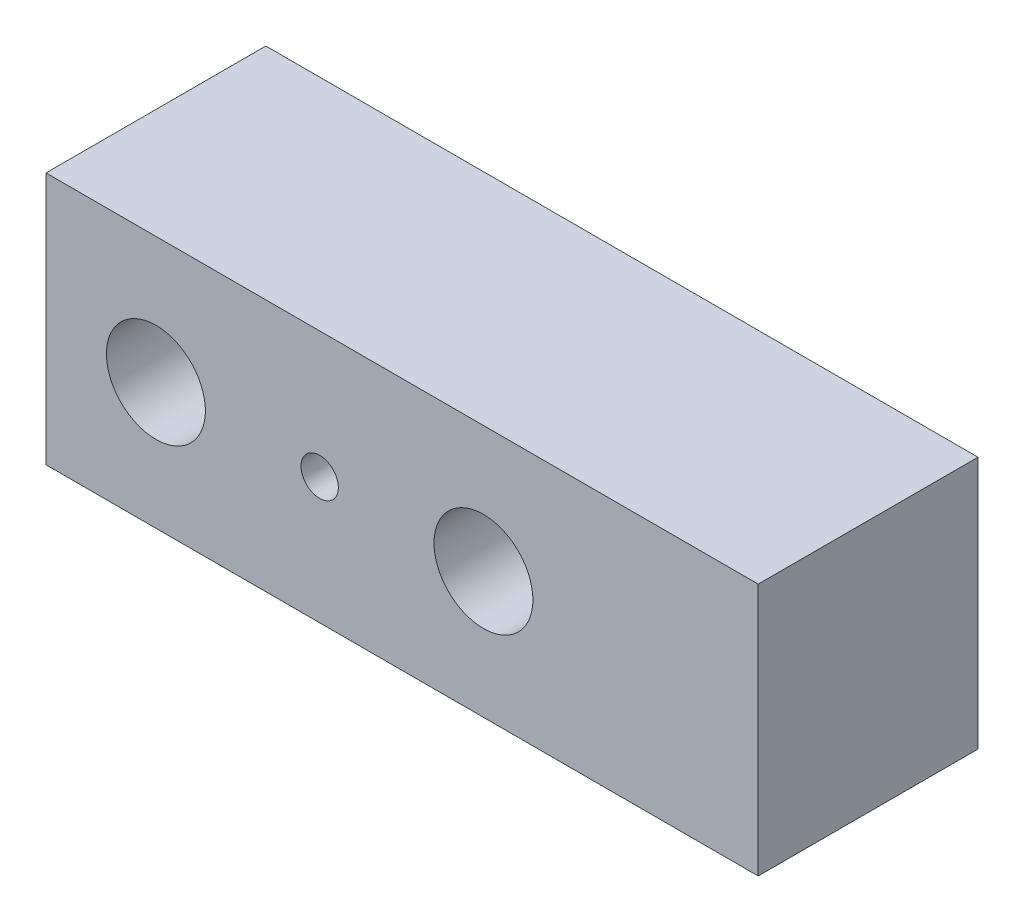
SolidWorks part; units mm, degrees
ref_plane "Front Plane" through (0, 0, 0) normal (0, 0, 1) x (1, 0, 0)
ref_plane "Top Plane" through (0, 0, 0) normal (0, 1, 0) x (1, 0, 0)
ref_plane "Right Plane" through (0, 0, 0) normal (1, 0, 0) x (0, 0, -1)
sketch "Sketch1" plane through (0, 0, 0) normal (0, 1, 0) x (1, 0, 0)
  line L1 (32.4, 10) -> (-32.4, 10)
  line L2 (32.4, 10) -> (32.4, -10)
  line L3 (32.4, -10) -> (-32.4, -10)
  line L4 (-32.4, 10) -> (-32.4, -10)
  line L5 (32.4, 10) -> (-32.4, -10) construction
  line L6 (32.4, -10) -> (-32.4, 10) construction
  point P0 (0, 0)
  dimension "D1" = 64.8
  dimension "D2" = 20
extrude "Boss-Extrude1" add sketch "Sketch1" along normal blind 23
sketch "Sketch2" plane through (0, 0, 0) normal (0, 1, 0) x (1, 0, 0)
  line L0 (-32.4, -10) -> (32.4, -10) construction
  circle A13 centre (18.9, -6) radius 1.5
  point P2 (24.836, -6)
  dimension "D1" = 3
  dimension "D2" = 4
extrude "Cut-Extrude1" cut sketch "Sketch2" along normal blind 20
sketch "Sketch3" plane through (0, 0, -10) normal (0, 0, -1) x (-1, 0, 0)
  line L2 (-17.4, 0) -> (-17.4, 20) construction
  line L3 (32.4, 23) -> (32.4, 0) construction
  line L4 (22.4, 11.5) -> (-7.4, 11.5) construction
  circle A0 centre (22.4, 11.5) radius 3.6669
  circle A1 centre (-7.4, 11.5) radius 3.6669
  circle A2 centre (7.5, 11.5) radius 3.3898
  point P10 (7.5, 11.5)
  dimension "D1" = 10
  dimension "D2" = 10
hole_wizard "CBORE for M8 Hex Socket Head Cap Screw1" positions "3DSketch2" profile "Sketch4" counterbore size "M8" standard "ISO"
sketch3d "3DSketch2"
  point P0 (-22.4, 11.5, -10)
  point P3 (-22.4, 11.5, -10)
  point P5 (7.4, 11.5, -10)
  point P8 (7.4, 11.5, -10)
  point P10 (7.4, 11.5, -10)
sketch "Sketch4" plane through (-22.4, 11.5, -10) normal (1, 0, 0) x (0, 1, 0)
  line L0 (0, 0) -> (0, 44.6439)
  line L1 (0, 44.6439) -> (4.5, 41.94)
  line L2 (4.5, 41.94) -> (4.5, 8.6)
  line L3 (4.5, 8.6) -> (7.5, 8.6)
  line L4 (7.5, 8.6) -> (7.5, 0)
  line L5 (7.5, 0) -> (0, 0)
  line L10 (0, 44.6439) -> (-4.5, 41.94) construction
  line L11 (0, -6.35) -> (0, 107.95) construction
  dimension "Hole Dia." = 9
  dimension "Hole Depth" = 41.94
  dimension "C'Bore Dia." = 15
  dimension "C'Bore Depth" = 8.6
  dimension "Drill Angle" = 118
hole_wizard "CBORE for M3 Hex Socket Head Cap Screw1" positions "3DSketch3" profile "Sketch5" counterbore size "M3" standard "ISO"
sketch3d "3DSketch3"
  point P0 (-7.5, 11.5, -10)
sketch "Sketch5" plane through (-7.5, 11.5, -10) normal (1, 0, 0) x (0, 1, 0)
  line L0 (0, 0) -> (0, 42.9615)
  line L1 (0, 42.9615) -> (1.7, 41.94)
  line L2 (1.7, 41.94) -> (1.7, 3.4)
  line L3 (1.7, 3.4) -> (3.25, 3.4)
  line L4 (3.25, 3.4) -> (3.25, 0)
  line L5 (3.25, 0) -> (0, 0)
  line L10 (0, 42.9615) -> (-1.7, 41.94) construction
  line L11 (0, -6.35) -> (0, 107.95) construction
  dimension "Hole Dia." = 3.4
  dimension "Hole Depth" = 41.94
  dimension "C'Bore Dia." = 6.5
  dimension "C'Bore Depth" = 3.4
  dimension "Drill Angle" = 118
